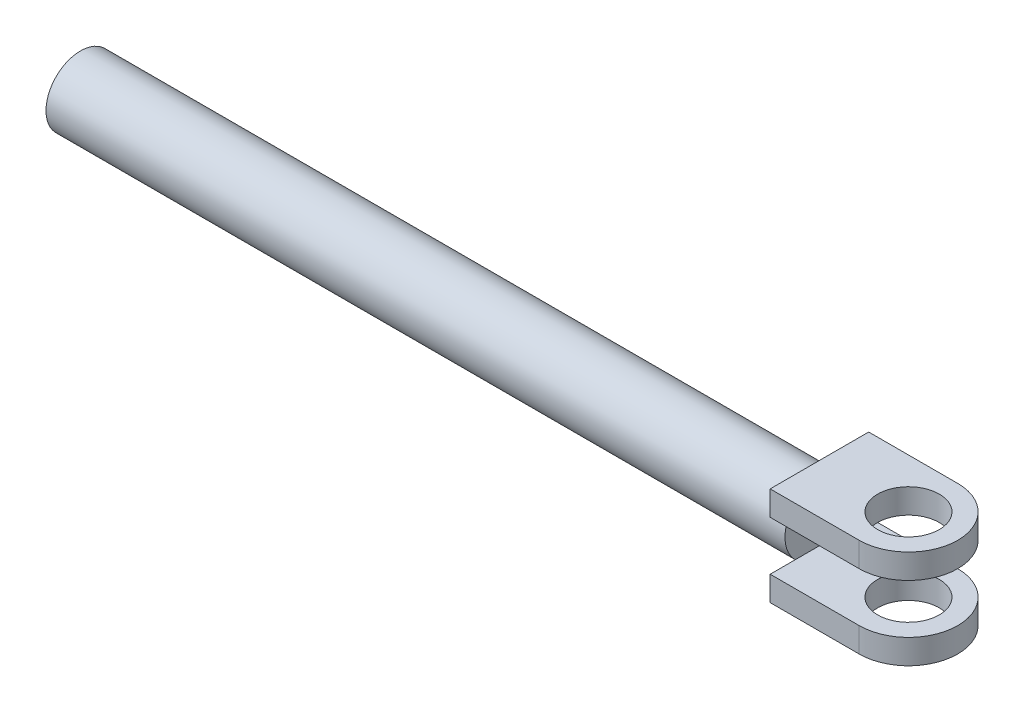
SolidWorks part; units mm, degrees
ref_plane "Front Plane" through (0, 0, 0) normal (0, 0, 1) x (1, 0, 0)
ref_plane "Top Plane" through (0, 0, 0) normal (0, 1, 0) x (1, 0, 0)
ref_plane "Right Plane" through (0, 0, 0) normal (1, 0, 0) x (0, 0, -1)
other "Configuration Table"
sketch "Sketch1" plane through (0, 0, 0) normal (0, 1, 0) x (1, 0, 0)
  line L0 (0, 0) -> (72.2857, 0) construction
  line L1 (36.1429, 20) -> (72.2857, 20)
  line L2 (36.1429, -20) -> (72.2857, -20)
  line L3 (36.1429, 20) -> (36.1429, -20)
  arc A1 (72.2857, -20) -> (72.2857, 20) centre (72.2857, 0) ccw
  circle A2 centre (72.2857, 0) radius 12.5
  point P3 (36.1429, 0)
  dimension "D1" = 20
  dimension "D2" = 25
extrude "Boss-Extrude1" add sketch "Sketch1" along normal blind 10
sketch "Sketch2" plane through (36.1429, 0, 0) normal (-1, 0, 0) x (0, 0, 1)
  line L0 (0, 0) -> (0, -10) construction
  line L1 (-20, 0) -> (20, 0) construction
  circle A0 centre (0, -10) radius 14
  dimension "D2" = 28
  dimension "D1" = 10
extrude "Boss-Extrude2" add sketch "Sketch2" along normal blind 300
ref_plane "Plane1" through (0, -10, 0) normal (0, -1, 0) x (-1, 0, 0)
mirror "Mirror1" about plane through (0, -10, 0) normal (0, -1, 0) of "Boss-Extrude1"
